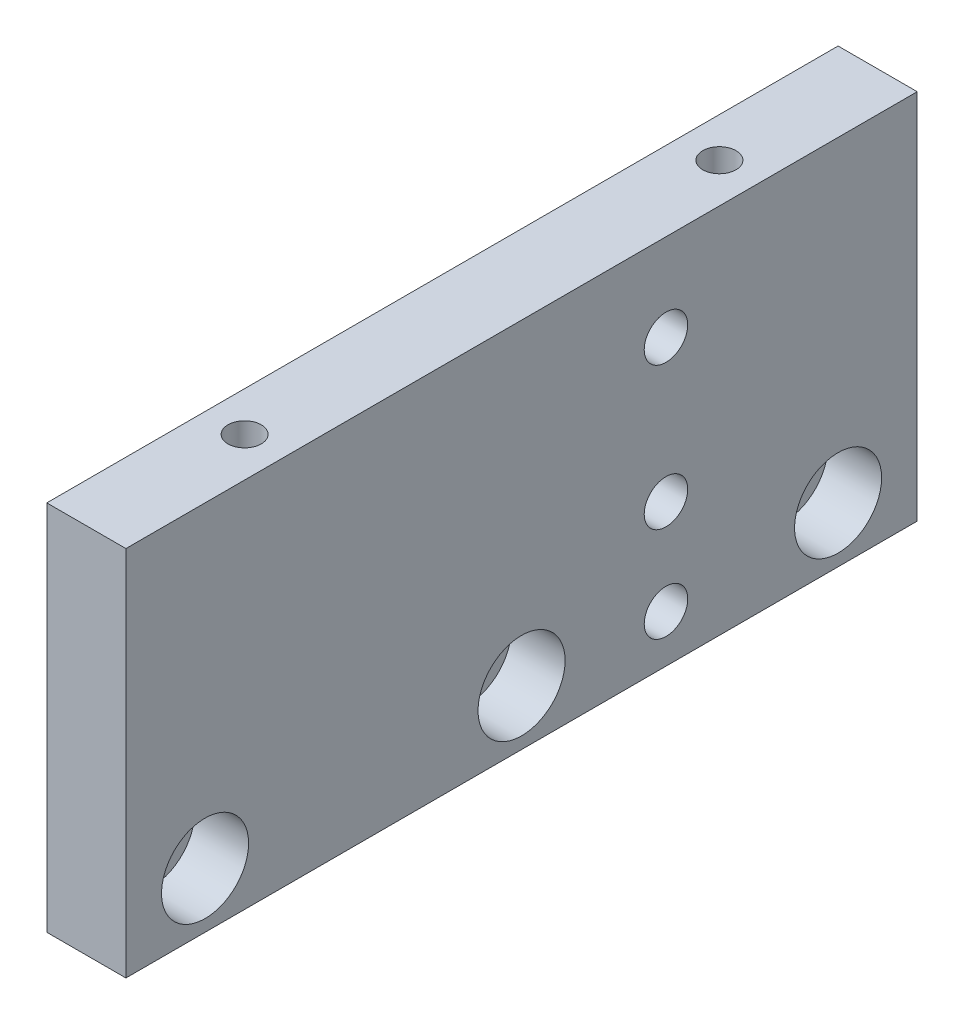
SolidWorks part; units mm, degrees
ref_plane "前视基准面" through (0, 0, 0) normal (0, 0, 1) x (1, 0, 0)
ref_plane "上视基准面" through (0, 0, 0) normal (0, 1, 0) x (1, 0, 0)
ref_plane "右视基准面" through (0, 0, 0) normal (1, 0, 0) x (0, 0, -1)
sketch "草图1" plane through (0, 0, 0) normal (1, 0, 0) x (0, 0, -1)
  line L1 (-50, 23.5) -> (50, 23.5)
  line L2 (-50, 23.5) -> (-50, -23.5)
  line L3 (-50, -23.5) -> (50, -23.5)
  line L4 (50, 23.5) -> (50, -23.5)
  line L5 (-50, 23.5) -> (50, -23.5) construction
  line L6 (-50, -23.5) -> (50, 23.5) construction
  point P0 (0, 0)
  dimension "D1" = 100
  dimension "D2" = 47
extrude "凸台-拉伸1" add sketch "草图1" along normal blind 10
hole_wizard "打孔尺寸(%根据)内六角圆柱头螺钉的类型1" positions "草图2" profile "草图3" counterbore size "M6" standard "GB"
sketch "草图2" plane through (10, 0, 0) normal (1, 0, 0) x (0, 0, -1)
  line L0 (0, 0) -> (0, -59.6587) construction
  line L2 (-50, -23.5) -> (50, -23.5) construction
  point P0 (-40, -16.5)
  point P2 (0, -16.5)
  point P4 (40, -16.5)
  dimension "D1" = 80
  dimension "D2" = 7
sketch "草图3" plane through (10, -16.5, 40) normal (0, 1, 0) x (0, 0, -1)
  line L0 (0, 0) -> (0, 16.9828)
  line L1 (0, 16.9828) -> (3.3, 15)
  line L2 (3.3, 15) -> (3.3, 6.8)
  line L3 (3.3, 6.8) -> (5.5, 6.8)
  line L4 (5.5, 6.8) -> (5.5, 0)
  line L5 (5.5, 0) -> (0, 0)
  line L10 (0, 16.9828) -> (-3.3, 15) construction
  line L11 (0, -6.35) -> (0, 107.95) construction
  dimension "孔直径" = 6.6
  dimension "孔深度" = 15
  dimension "柱形沉头孔直径" = 11
  dimension "柱形沉头孔深度" = 6.8
  dimension "导头角度" = 118
hole_wizard "打孔尺寸(%根据)内六角圆柱头螺钉的类型2" positions "草图4" profile "草图5" counterbore size "M5" standard "GB" end condition through all
sketch "草图4" plane through (0, 0, 0) normal (-1, 0, 0) x (0, 0, 1)
  line L0 (50, -23.5) -> (-50, -23.5) construction
  line L1 (-50, -23.5) -> (-50, 23.5) construction
  point P0 (-18.25, 12.5)
  point P2 (-18.25, -5.5)
  point P4 (-18.25, -17.5)
  dimension "D1" = 18
  dimension "D2" = 12
  dimension "D3" = 6
  dimension "D4" = 31.75
sketch "草图5" plane through (0, 12.5, -18.25) normal (0, 1, 0) x (0, 0, 1)
  line L0 (0, 0) -> (0, 10)
  line L1 (0, 10) -> (2.75, 10)
  line L3 (2.75, 10) -> (2.75, 5.7)
  line L4 (2.75, 5.7) -> (5, 5.7)
  line L5 (5, 5.7) -> (5, 0)
  line L7 (5, 0) -> (0, 0)
  line L11 (0, -6.35) -> (0, 107.95) construction
  dimension "通孔孔直径" = 5.5
  dimension "通孔孔深度" = 10
  dimension "柱形沉头孔直径" = 10
  dimension "柱形沉头孔深度" = 5.7
hole_wizard "M5 螺纹孔1" positions "草图6" profile "草图7" tap size "M5" standard "GB"
sketch "草图6" plane through (0, 23.5, 0) normal (0, 1, 0) x (1, 0, 0)
  line L0 (5, -50) -> (5, 52.4158) construction
  line L1 (10, -50) -> (0, -50) construction
  line L3 (1.3545, 0) -> (19.8774, 0) construction
  point P0 (5, -30)
  point P2 (5, 30)
  dimension "D1" = 60
sketch "草图7" plane through (5, 23.5, 30) normal (1, 0, 0) x (0, 0, 1)
  line L0 (0, 0) -> (0, 13.6618)
  line L1 (0, 13.6618) -> (2.1, 12.4)
  line L2 (2.1, 12.4) -> (2.1, 0)
  line L5 (2.1, 0) -> (0, 0)
  line L10 (0, 13.6618) -> (-2.1, 12.4) construction
  line L11 (0, -6.35) -> (0, 107.95) construction
  dimension "螺纹孔钻头直径" = 4.2
  dimension "螺纹孔钻头深度" = 12.4
  dimension "导头角度" = 118
cosmetic thread "孔螺蚊线1"
cosmetic thread "孔螺蚊线2"
